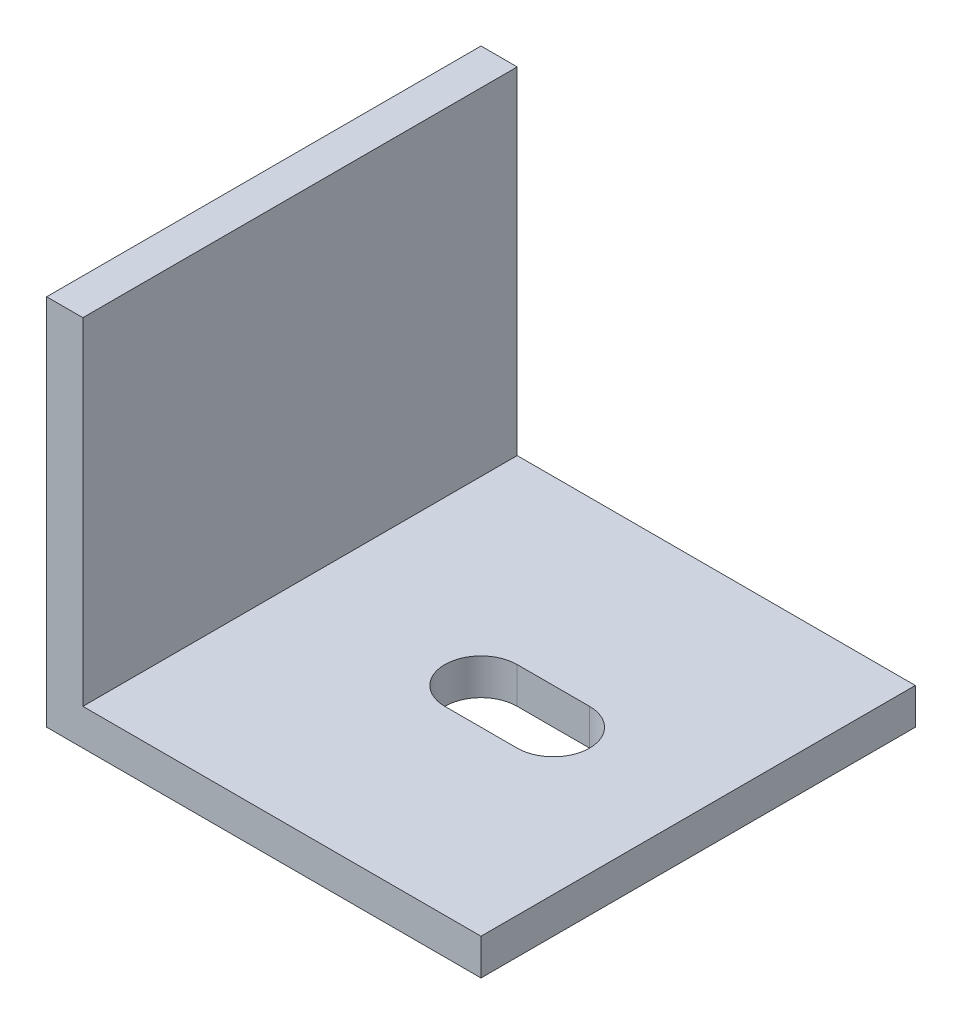
SolidWorks part; units mm, degrees
ref_plane "Front Plane" through (0, 0, 0) normal (0, 0, 1) x (1, 0, 0)
ref_plane "Top Plane" through (0, 0, 0) normal (0, 1, 0) x (1, 0, 0)
ref_plane "Right Plane" through (0, 0, 0) normal (1, 0, 0) x (0, 0, -1)
other "Configuration Table"
sketch "Sketch1" plane through (0, 0, 0) normal (0, 0, 1) x (1, 0, 0)
  line L0 (0, 0) -> (0, 103)
  line L1 (0, 0) -> (120, 0)
  dimension "D1" = 120
  dimension "D2" = 103
extrude "Extrude-Thin1" add sketch "Sketch1" along normal mid plane 120 thin
sketch "Sketch2" plane through (0, 10, 0) normal (0, 1, 0) x (1, 0, 0)
  line L0 (60, 0) -> (80, 0) construction
  line L1 (60, 10) -> (80, 10)
  line L2 (60, -10) -> (80, -10)
  line L3 (120, -60) -> (120, 60) construction
  arc A0 (60, 10) -> (60, -10) centre (60, 0) ccw
  arc A1 (80, -10) -> (80, 10) centre (80, 0) ccw
  point P3 (70, 0)
  dimension "D1" = 10
  dimension "D2" = 40
  dimension "D3" = 20
extrude "Cut-Extrude1" cut sketch "Sketch2" against normal through all
